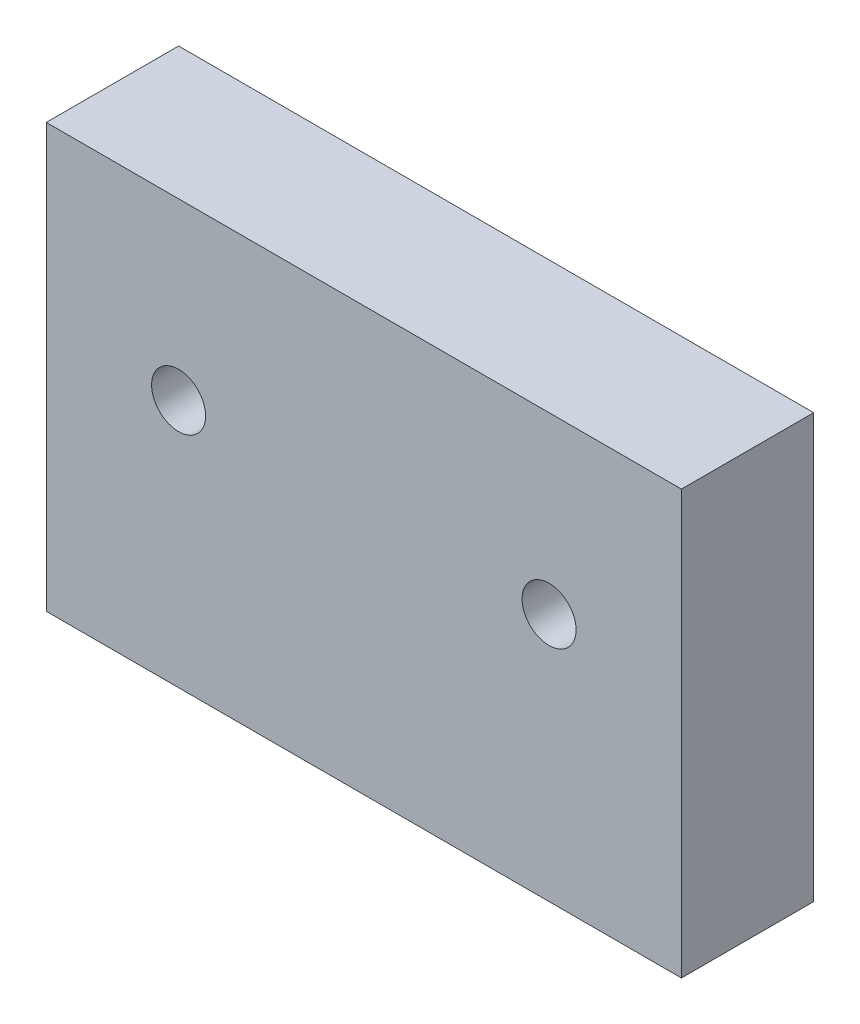
SolidWorks part; units mm, degrees
material "1023 碳钢板 (SS)"
ref_plane "Front Plane" through (0, 0, 0) normal (0, 0, 1) x (1, 0, 0)
ref_plane "Top Plane" through (0, 0, 0) normal (0, 1, 0) x (1, 0, 0)
ref_plane "Right Plane" through (0, 0, 0) normal (1, 0, 0) x (0, 0, -1)
sketch "Sketch1" plane through (0, 0, 0) normal (0, 0, 1) x (1, 0, 0)
  line L1 (60, 40) -> (-60, 40)
  line L2 (60, 40) -> (60, -40)
  line L3 (60, -40) -> (-60, -40)
  line L4 (-60, 40) -> (-60, -40)
  line L5 (60, 40) -> (-60, -40) construction
  line L6 (60, -40) -> (-60, 40) construction
  point P0 (0, 0)
  dimension "D1" = 120
  dimension "D2" = 80
extrude "Boss-Extrude1" add sketch "Sketch1" along normal blind 25
sketch "Sketch2" plane through (0, 0, 25) normal (0, 0, 1) x (1, 0, 0)
  line L0 (60, 40) -> (-60, 40) construction
  circle A0 centre (-35, 7) radius 4.5
  circle A1 centre (35, 7) radius 4.5
  dimension "D4" = 9
  dimension "D1" = 70
  dimension "D2" = 35
  dimension "D3" = 33
hole_wizard "M12 Tapped Hole1" positions "Sketch3" profile "Sketch4" tap size "M12" standard "ISO"
sketch "Sketch3" plane through (0, 0, 25) normal (0, 0, 1) x (1, 0, 0)
  point P0 (-35, 7)
  point P3 (35, 7)
sketch "Sketch4" plane through (-35, 7, 25) normal (1, 0, 0) x (0, -1, 0)
  line L0 (0, 0) -> (0, 32.3144)
  line L1 (0, 32.3144) -> (5.1, 29.25)
  line L2 (5.1, 29.25) -> (5.1, 0)
  line L5 (5.1, 0) -> (0, 0)
  line L10 (0, 32.3144) -> (-5.1, 29.25) construction
  line L11 (0, -6.35) -> (0, 107.95) construction
  dimension "螺纹孔钻头直径" = 10.2
  dimension "螺纹孔钻头深度" = 29.25
  dimension "导头角度" = 118
cosmetic thread "Hole Thread Line 1" parameters "D1"=24, "D2"=12
cosmetic thread "Hole Thread Line 2" parameters "D1"=24, "D2"=12
